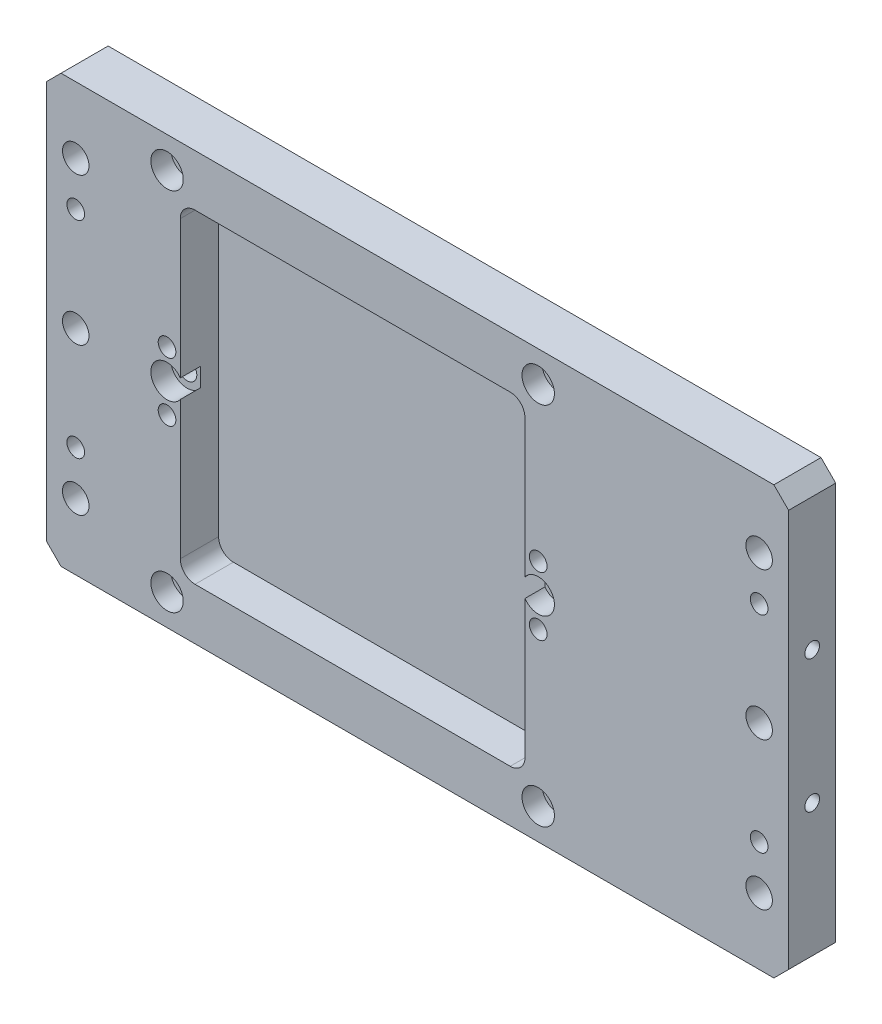
SolidWorks part; units mm, degrees
material "AL6061"
ref_plane "前视基准面" through (0, 0, 0) normal (0, 0, 1) x (1, 0, 0)
ref_plane "上视基准面" through (0, 0, 0) normal (0, 1, 0) x (1, 0, 0)
ref_plane "右视基准面" through (0, 0, 0) normal (1, 0, 0) x (0, 0, -1)
sketch "草图1" plane through (0, 0, 0) normal (0, 0, 1) x (1, 0, 0)
  line L0 (-112.4601, 0) -> (116.8053, 0) construction
  line L1 (0, 64.0136) -> (0, -65.8827) construction
  line L3 (-126, 72.5) -> (126, 72.5)
  line L4 (-126, 72.5) -> (-126, -72.5)
  line L5 (-126, -72.5) -> (126, -72.5)
  line L6 (126, 72.5) -> (126, -72.5)
  dimension "D1" = 252
  dimension "D2" = 145
extrude "凸台-拉伸1" add sketch "草图1" along normal mid plane 16
hole_wizard "打孔尺寸(%根据)内六角圆柱头螺钉的类型2" positions "草图2" profile "草图3" counterbore size "M6" standard "GB" end condition through all
sketch "草图2" plane through (0, 0, 8) normal (0, 0, 1) x (1, 0, 0)
  line L0 (-102.3868, 0) -> (104.6914, 0) construction
  line L3 (-22, 80.3531) -> (-22, -85.8193) construction
  line L4 (126, -72.5) -> (126, 72.5) construction
  point P0 (-85, 62)
  point P2 (-85, 0)
  point P6 (41, 62)
  point P8 (41, 0)
  point P14 (41, -62)
  point P15 (-85, -62)
  dimension "D1" = 148
  dimension "D2" = 126
  dimension "D3" = 124
sketch "草图3" plane through (-85, 62, 8) normal (1, 0, 0) x (0, -1, 0)
  line L0 (0, 0) -> (0, 16)
  line L1 (0, 16) -> (3.3, 16)
  line L3 (3.3, 16) -> (3.3, 6.8)
  line L4 (3.3, 6.8) -> (5.5, 6.8)
  line L5 (5.5, 6.8) -> (5.5, 0)
  line L7 (5.5, 0) -> (0, 0)
  line L11 (0, -6.35) -> (0, 107.95) construction
  dimension "通孔孔直径" = 6.6
  dimension "通孔孔深度" = 16
  dimension "柱形沉头孔直径" = 11
  dimension "柱形沉头孔深度" = 6.8
hole_wizard "打孔尺寸(%根据)内六角圆柱头螺钉的类型2" positions "草图4" profile "草图5" counterbore size "M8" standard "GB" end condition through all
sketch "草图4" plane through (0, 0, -8) normal (0, 0, -1) x (-1, 0, 0)
  line L0 (0, 65.4964) -> (0, -64.6476) construction
  line L1 (-129.0667, 0) -> (132.5867, 0) construction
  line L2 (-126, -72.5) -> (-126, 72.5) construction
  point P0 (-116, -50)
  point P2 (-116, 0)
  point P14 (-116, 50)
  dimension "D1" = 100
  dimension "D2" = 10
sketch "草图5" plane through (116, -50, -8) normal (1, 0, 0) x (0, 1, 0)
  line L0 (0, 0) -> (0, 16)
  line L1 (0, 16) -> (4.5, 16)
  line L3 (4.5, 16) -> (4.5, 9)
  line L4 (4.5, 9) -> (7.5, 9)
  line L5 (7.5, 9) -> (7.5, 0)
  line L7 (7.5, 0) -> (0, 0)
  line L11 (0, -6.35) -> (0, 107.95) construction
  dimension "通孔孔直径" = 9
  dimension "通孔孔深度" = 16
  dimension "柱形沉头孔直径" = 15
  dimension "柱形沉头孔深度" = 9
hole_wizard "Ø6.0 (6) 直径孔1" positions "草图6" profile "草图7" hole size "Ø6.0" standard "GB" end condition through all
sketch "草图6" plane through (0, 0, -8) normal (0, 0, -1) x (-1, 0, 0)
  line L0 (-126.3855, 0) -> (24.7303, 0) construction
  line L1 (-116, 0) -> (-116, 50) construction
  point P0 (-116, -35)
  point P7 (-116, 35)
  dimension "D1" = 70
sketch "草图7" plane through (116, -35, -8) normal (1, 0, 0) x (0, 1, 0)
  line L0 (0, 0) -> (0, 16)
  line L1 (0, 16) -> (3, 16)
  line L2 (3, 16) -> (3, 0)
  line L5 (3, 0) -> (0, 0)
  line L11 (0, -6.35) -> (0, 107.95) construction
  dimension "通孔孔直径" = 6
  dimension "通孔孔深度" = 16
mirror "镜向1" about plane through (0, 0, 0) normal (1, 0, 0) of "Ø6.0 (6) 直径孔1", "打孔尺寸(%根据)内六角圆柱头螺钉的类型2"
hole_wizard "Ø6.0 (6) 直径孔2" positions "草图8" profile "草图9" hole size "Ø6.0" standard "GB" end condition through all
sketch "草图8" plane through (0, 0, 8) normal (0, 0, 1) x (1, 0, 0)
  line L0 (41, 0) -> (41, -62) construction
  line L1 (-85, 0) -> (-85, -62) construction
  line L2 (-133.9978, 0) -> (130.2018, 0) construction
  point P0 (41, -10)
  point P18 (-85, -10)
  point P21 (-85, 10)
  point P22 (41, 10)
  dimension "D1" = 20
sketch "草图9" plane through (41, -10, 8) normal (1, 0, 0) x (0, -1, 0)
  line L0 (0, 0) -> (0, 16)
  line L1 (0, 16) -> (3, 16)
  line L2 (3, 16) -> (3, 0)
  line L5 (3, 0) -> (0, 0)
  line L11 (0, -6.35) -> (0, 107.95) construction
  dimension "通孔孔直径" = 6
  dimension "通孔孔深度" = 16
sketch "草图10" plane through (0, 0, 8) normal (0, 0, 1) x (1, 0, 0)
  line L0 (-133.5575, 0) -> (158.702, 0) construction
  line L1 (-22, 82.1752) -> (-22, -86.1837) construction
  line L3 (-75.5, 55) -> (31.5, 55)
  line L4 (-80.5, 50) -> (-80.5, -50)
  line L5 (-75.5, -55) -> (31.5, -55)
  line L6 (36.5, 50) -> (36.5, -50)
  circle A0 centre (-85, 62) radius 3.3 construction
  circle A1 centre (41, 62) radius 3.3 construction
  arc A2 (31.5, 55) -> (36.5, 50) centre (31.5, 50) cw
  arc A3 (-80.5, -50) -> (-75.5, -55) centre (-75.5, -50) ccw
  arc A4 (31.5, -55) -> (36.5, -50) centre (31.5, -50) ccw
  arc A5 (-75.5, 55) -> (-80.5, 50) centre (-75.5, 50) ccw
  dimension "D1" = 5
  dimension "D2" = 117
  dimension "D3" = 110
extrude "切除-拉伸1" cut sketch "草图10" against normal blind 13
chamfer "倒角1" distance 5 angle 45 4 edges at (-126, -72.5, 0) (126, -72.5, 0) (126, 72.5, 0) (-126, 72.5, 0)
hole_wizard "M6 螺纹孔2" positions "草图13" profile "草图14" tap size "M6" standard "ISO"
sketch "草图13" plane through (126, 0, 0) normal (1, 0, 0) x (0, 0, -1)
  line L0 (0, -64.8191) -> (0, 51.4581) construction
  line L1 (-11.3749, 0) -> (11.5555, 0) construction
  point P0 (0, 22.5)
  point P9 (0, -22.5)
  dimension "D1" = 45
sketch "草图14" plane through (126, 22.5, 0) normal (0, 1, 0) x (0, 0, -1)
  line L0 (0, 0) -> (0, 24.5022)
  line L1 (0, 24.5022) -> (2.5, 23)
  line L2 (2.5, 23) -> (2.5, 0)
  line L5 (2.5, 0) -> (0, 0)
  line L10 (0, 24.5022) -> (-2.5, 23) construction
  line L11 (0, -6.35) -> (0, 107.95) construction
  dimension "螺纹孔钻头直径" = 5
  dimension "螺纹孔钻头深度" = 23
  dimension "导头角度" = 118
cosmetic thread "孔螺蚊线3" parameters "D1"=20, "D2"=6
cosmetic thread "孔螺蚊线4" parameters "D1"=20, "D2"=6
